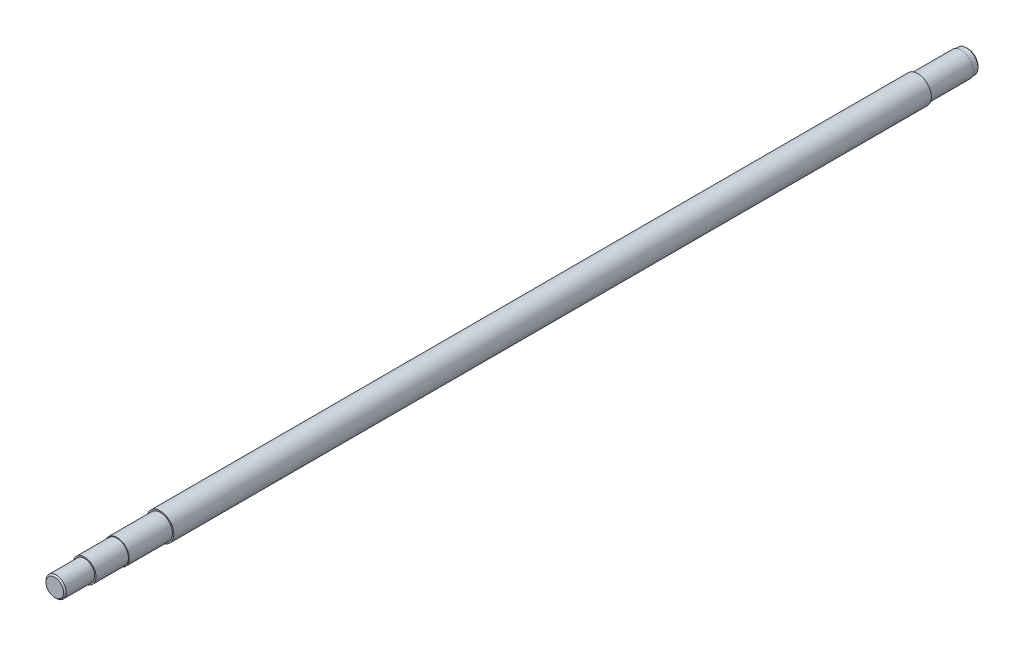
from build123d import *

# Parameters (mm, degrees)
SKETCH_1_R          = 37.5
EXTRUDE_1_DEPTH     = 140
SKETCH_2_R          = 42.5
EXTRUDE_2_DEPTH     = 120
SKETCH_3_R          = 45
EXTRUDE_3_DEPTH     = 160
SKETCH_4_R          = 50
EXTRUDE_4_DEPTH     = 2800
SKETCH_5_R          = 45
EXTRUDE_5_DEPTH     = 160
SKETCH_6_R          = 42.5
EXTRUDE_6_DEPTH     = 120
SKETCH_7_R          = 37.5
EXTRUDE_7_DEPTH     = 110
SKETCH_8_R          = 75
CUT_EXTRUDE_1_DEPTH = 235
CHAMFER_1_SIZE      = 5


with BuildPart() as part:
    # 草图1 → 凸台-拉伸1 (new body)
    with BuildSketch(Plane.XY):
        Circle(SKETCH_1_R)
    extrude(amount=EXTRUDE_1_DEPTH)

    # 草图2 → 凸台-拉伸2 (add)
    with BuildSketch(Plane.XY.offset(140)):
        Circle(SKETCH_2_R)
    extrude(amount=EXTRUDE_2_DEPTH)

    # 草图3 → 凸台-拉伸3 (add)
    with BuildSketch(Plane.XY.offset(260)):
        Circle(SKETCH_3_R)
    extrude(amount=EXTRUDE_3_DEPTH)

    # 草图4 → 凸台-拉伸4 (add)
    with BuildSketch(Plane.XY.offset(420)):
        Circle(SKETCH_4_R)
    extrude(amount=EXTRUDE_4_DEPTH)

    # 草图5 → 凸台-拉伸5 (add)
    with BuildSketch(Plane.XY.offset(3220)):
        Circle(SKETCH_5_R)
    extrude(amount=EXTRUDE_5_DEPTH)

    # 草图6 → 凸台-拉伸6 (add)
    with BuildSketch(Plane.XY.offset(3380)):
        Circle(SKETCH_6_R)
    extrude(amount=EXTRUDE_6_DEPTH)

    # 草图7 → 凸台-拉伸7 (add)
    with BuildSketch(Plane.XY.offset(3500)):
        Circle(SKETCH_7_R)
    extrude(amount=EXTRUDE_7_DEPTH)

    # 草图8 → 切除-拉伸1 (cut)
    with BuildSketch(Plane(origin=(0, 0, 0), x_dir=(-1, 0, 0), z_dir=(0, 0, -1))):
        Circle(SKETCH_8_R)
    extrude(amount=-CUT_EXTRUDE_1_DEPTH, mode=Mode.SUBTRACT)

    # 倒角1
    chamfer_1_edges = [part.edges().sort_by_distance(p)[0] for p in [
        (-37.5, 0, 3610),
        (-42.5, 0, 235),
    ]]
    chamfer(chamfer_1_edges, length=CHAMFER_1_SIZE)


solid = part.part
